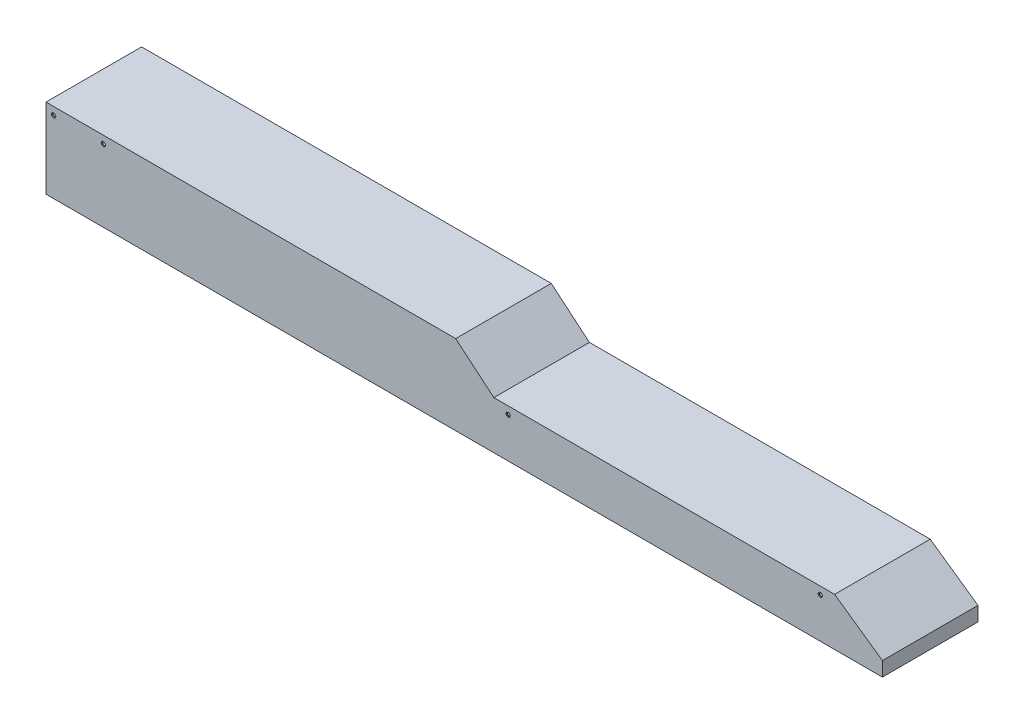
from build123d import *

# Parameters (mm, degrees)
EXTRUDE_1_DEPTH        = 100
SHELL_1_T              = -2
SKETCH_2_W             = 1750
SKETCH_2_H             = 200
SKETCH_2_W_2           = 1662
SKETCH_2_H_2           = 140
EXTRUDE_2_DEPTH        = 2
SKETCH_3_R             = 4.5
CUT_EXTRUDE_1_DEPTH    = 2
EXTRUDE_4_DEPTH        = 8
HOLE_WIZARD_M8_1_D     = 6.8
HOLE_WIZARD_M8_1_DEPTH = 19.75
HOLE_WIZARD_M8_1_TIP   = 2.042926105
SKETCH_8_R             = 4.5
CUT_EXTRUDE_2_DEPTH    = 8
EXTRUDE_5_DEPTH        = 8
HOLE_WIZARD_M8_2_D     = 6.8
HOLE_WIZARD_M8_2_DEPTH = 19.75
HOLE_WIZARD_M8_2_TIP   = 2.042926105


with BuildPart() as part:
    # 草图1 → 凸台-拉伸1 (new, symmetric)
    with BuildSketch(Plane.XY):
        Polygon((-1750, 0), (0, 0), (0, 30), (-99.970360472, 100), (-813, 100), (-892.847490704, 167), (-1750, 167), align=None)
    extrude(amount=EXTRUDE_1_DEPTH, both=True)

    # 抽壳1
    shell_1_openings = [part.faces().sort_by_distance(p)[0] for p in [
        (-875, 0, 0),
    ]]
    offset(amount=SHELL_1_T, openings=shell_1_openings, kind=Kind.INTERSECTION)

    # 草图2 → 凸台-拉伸2 (add)
    with BuildSketch(Plane.XZ):
        with Locations((-875, 0)):
            Rectangle(SKETCH_2_W, SKETCH_2_H)
        with Locations((-875, 0)):
            Rectangle(SKETCH_2_W_2, SKETCH_2_H_2, mode=Mode.SUBTRACT)
    extrude(amount=-EXTRUDE_2_DEPTH)

    # 草图3 → 切除-拉伸1 (cut)
    with BuildSketch(Plane.XZ):
        with Locations(Location((-1720, 84, 0), (0, 0, 270))):
            Circle(SKETCH_3_R)
        with Locations(Location((-1156.666666667, 84, 0), (0, 0, 270))):
            Circle(SKETCH_3_R)
        with Locations(Location((-593.333333333, 84, 0), (0, 0, 270))):
            Circle(SKETCH_3_R)
        with Locations(Location((-30, 84, 0), (0, 0, 270))):
            Circle(SKETCH_3_R)
        with Locations(Location((-30, -84, 0), (0, 0, 90))):
            Circle(SKETCH_3_R)
        with Locations(Location((-593.333333333, -84, 0), (0, 0, 90))):
            Circle(SKETCH_3_R)
        with Locations(Location((-1156.666666667, -84, 0), (0, 0, 90))):
            Circle(SKETCH_3_R)
        with Locations(Location((-1720, -84, 0), (0, 0, 90))):
            Circle(SKETCH_3_R)
    extrude(amount=-CUT_EXTRUDE_1_DEPTH, mode=Mode.SUBTRACT)

    # 草图4 → 凸台-拉伸4 (add)
    with BuildSketch(Plane(origin=(0, 2, 0), x_dir=(1, 0, 0), z_dir=(0, 1, 0))):
        Polygon((-1713.922957331, -87.508582221), (-1713.922957331, -80.491417779), (-1720, -76.982835559), (-1726.077042669, -80.491417779), (-1726.077042669, -87.508582221), (-1720, -91.017164441), align=None)
        Polygon((-1720, 92.703139603), (-1727.537139989, 88.351569801), (-1727.537139989, 79.648430199), (-1720, 75.296860397), (-1712.462860011, 79.648430199), (-1712.462860011, 88.351569801), align=None)
        Polygon((-1156.666666667, 92.703139603), (-1164.203806655, 88.351569801), (-1164.203806655, 79.648430199), (-1156.666666667, 75.296860397), (-1149.129526678, 79.648430199), (-1149.129526678, 88.351569801), align=None)
        Polygon((-1156.666666667, -76.982835559), (-1162.743709335, -80.491417779), (-1162.743709335, -87.508582221), (-1156.666666667, -91.017164441), (-1150.589623998, -87.508582221), (-1150.589623998, -80.491417779), align=None)
        Polygon((-593.333333333, -76.982835559), (-599.410376002, -80.491417779), (-599.410376002, -87.508582221), (-593.333333333, -91.017164441), (-587.256290665, -87.508582221), (-587.256290665, -80.491417779), align=None)
        Polygon((-30, -76.982835559), (-36.077042669, -80.491417779), (-36.077042669, -87.508582221), (-30, -91.017164441), (-23.922957331, -87.508582221), (-23.922957331, -80.491417779), align=None)
        Polygon((-30, 92.703139603), (-37.537139989, 88.351569801), (-37.537139989, 79.648430199), (-30, 75.296860397), (-22.462860011, 79.648430199), (-22.462860011, 88.351569801), align=None)
        Polygon((-593.333333333, 92.703139603), (-600.870473322, 88.351569801), (-600.870473322, 79.648430199), (-593.333333333, 75.296860397), (-585.796193345, 79.648430199), (-585.796193345, 88.351569801), align=None)
    extrude(amount=EXTRUDE_4_DEPTH)

    # M8 螺纹孔1
    with Locations(Plane.XZ):
        with Locations((-1720, 84), (-1720, -84), (-1156.666666667, -84), (-1156.666666667, 84), (-593.333333333, 84), (-593.333333333, -84), (-30, 84), (-30, -84)):
            Hole(HOLE_WIZARD_M8_1_D / 2, depth=HOLE_WIZARD_M8_1_DEPTH)
            with Locations((0, 0, -(HOLE_WIZARD_M8_1_DEPTH + HOLE_WIZARD_M8_1_TIP / 2))):  # 118° drill point
                Cone(0, HOLE_WIZARD_M8_1_D / 2, HOLE_WIZARD_M8_1_TIP, mode=Mode.SUBTRACT)

    # 草图8 → 切除-拉伸2 (cut)
    with BuildSketch(Plane.XY.offset(100)):
        with Locations((-1734, 151)):
            Circle(SKETCH_8_R)
        with Locations((-1630, 151)):
            Circle(SKETCH_8_R)
        with Locations((-783, 84)):
            Circle(SKETCH_8_R)
        with Locations((-129.970360472, 84)):
            Circle(SKETCH_8_R)
    extrude(amount=-CUT_EXTRUDE_2_DEPTH, mode=Mode.SUBTRACT)

    # 草图9 → 凸台-拉伸5 (add)
    with BuildSketch(Plane(origin=(0, 0, 98), x_dir=(-1, 0, 0), z_dir=(0, 0, -1))):
        Polygon((1630, 161.198993807), (1621.16741227, 156.099496903), (1621.16741227, 145.900503097), (1630, 140.801006193), (1638.83258773, 145.900503097), (1638.83258773, 156.099496903), align=None)
        Polygon((1734, 159.898147478), (1726.293978237, 155.449073739), (1726.293978237, 146.550926261), (1734, 142.101852522), (1741.706021763, 146.550926261), (1741.706021763, 155.449073739), align=None)
        Polygon((783, 90.89472697), (777.028991292, 87.447363485), (777.028991292, 80.552636515), (783, 77.10527303), (788.971008708, 80.552636515), (788.971008708, 87.447363485), align=None)
        Polygon((129.970360472, 92.674432694), (122.458081396, 88.337216347), (122.458081396, 79.662783653), (129.970360472, 75.325567306), (137.482639548, 79.662783653), (137.482639548, 88.337216347), align=None)
    extrude(amount=EXTRUDE_5_DEPTH)

    # M8 螺纹孔2
    with Locations(Plane.XY.offset(100)):
        with Locations((-1630, 151), (-1734, 151), (-783, 84), (-129.970360472, 84)):
            Hole(HOLE_WIZARD_M8_2_D / 2, depth=HOLE_WIZARD_M8_2_DEPTH)
            with Locations((0, 0, -(HOLE_WIZARD_M8_2_DEPTH + HOLE_WIZARD_M8_2_TIP / 2))):  # 118° drill point
                Cone(0, HOLE_WIZARD_M8_2_D / 2, HOLE_WIZARD_M8_2_TIP, mode=Mode.SUBTRACT)


solid = part.part
